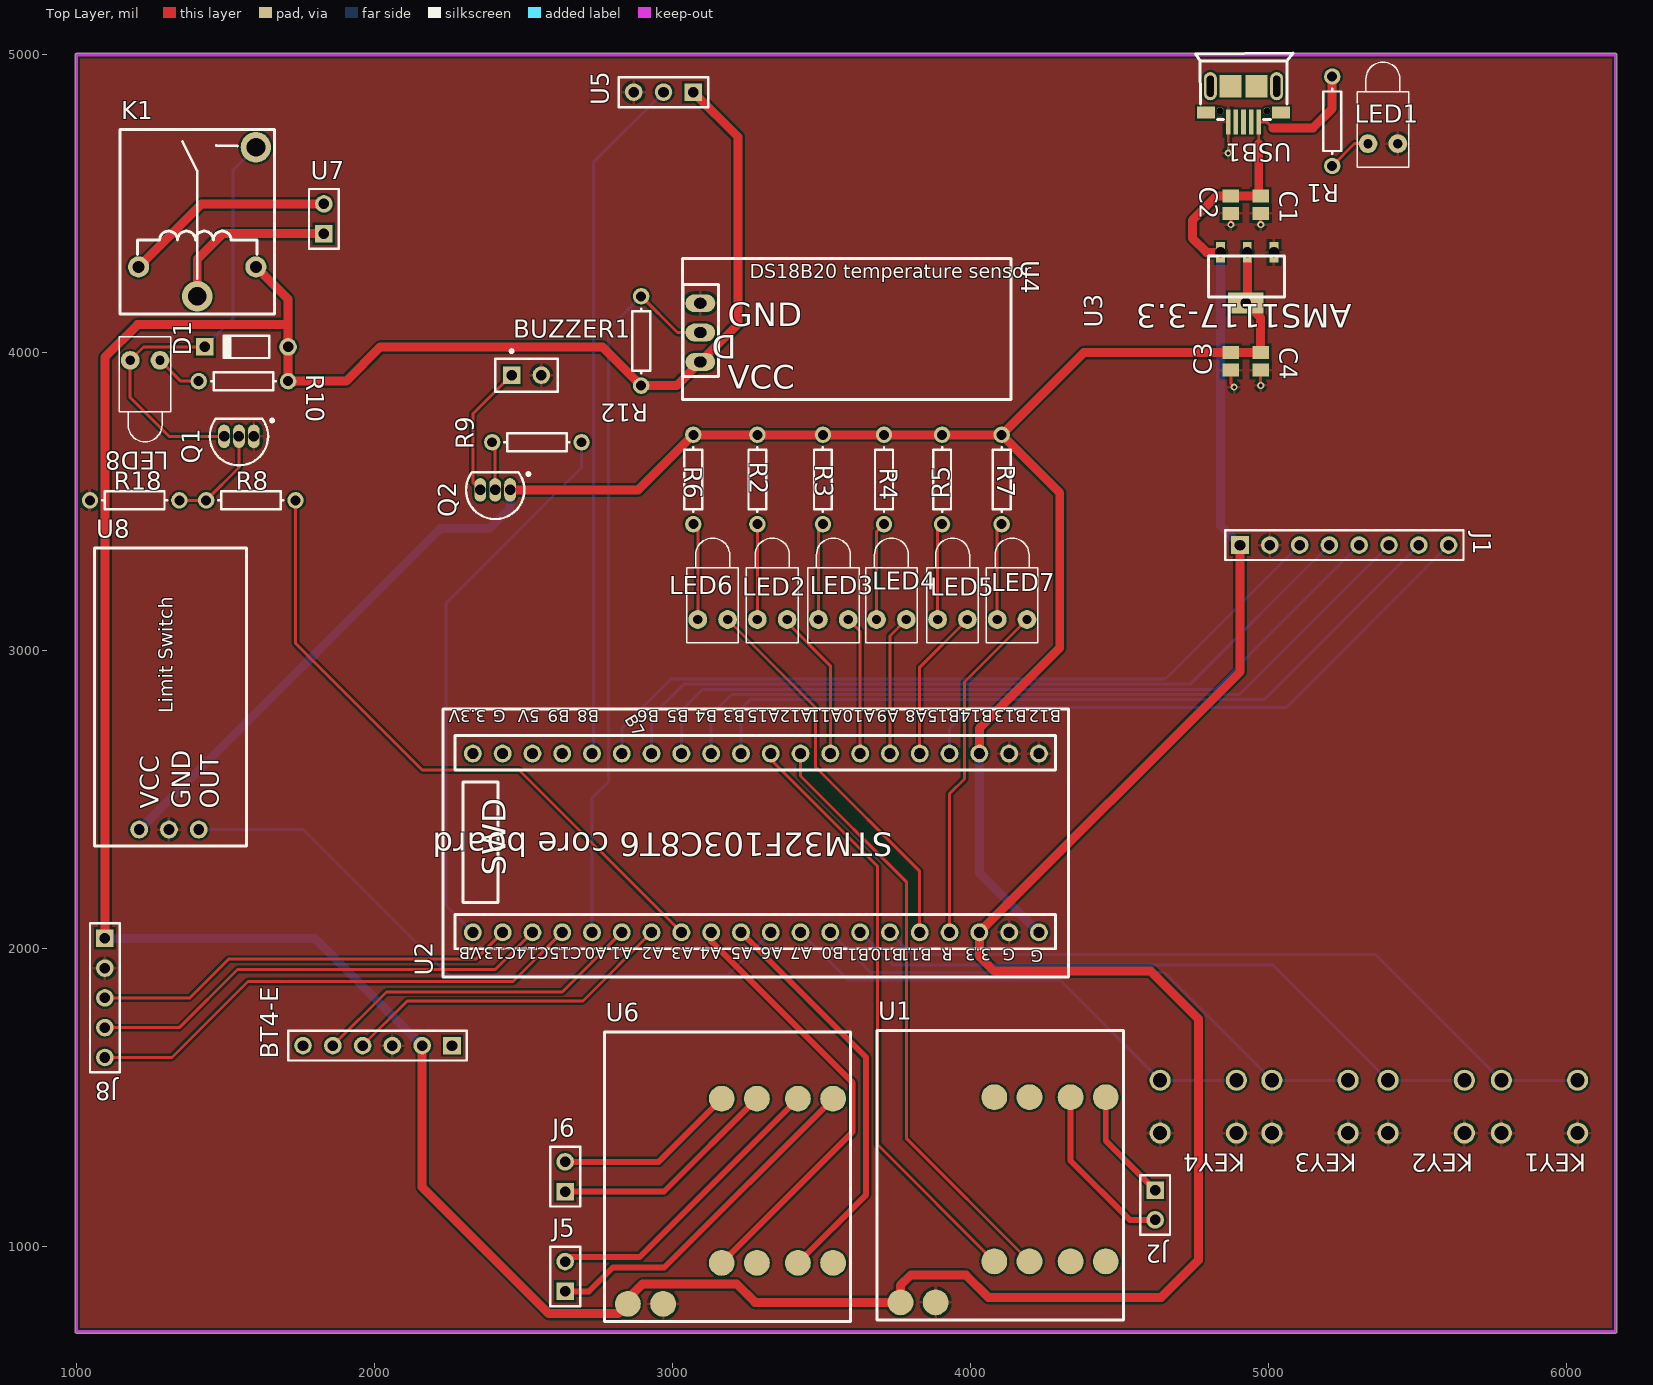
[diagram p0: Top Layer view]
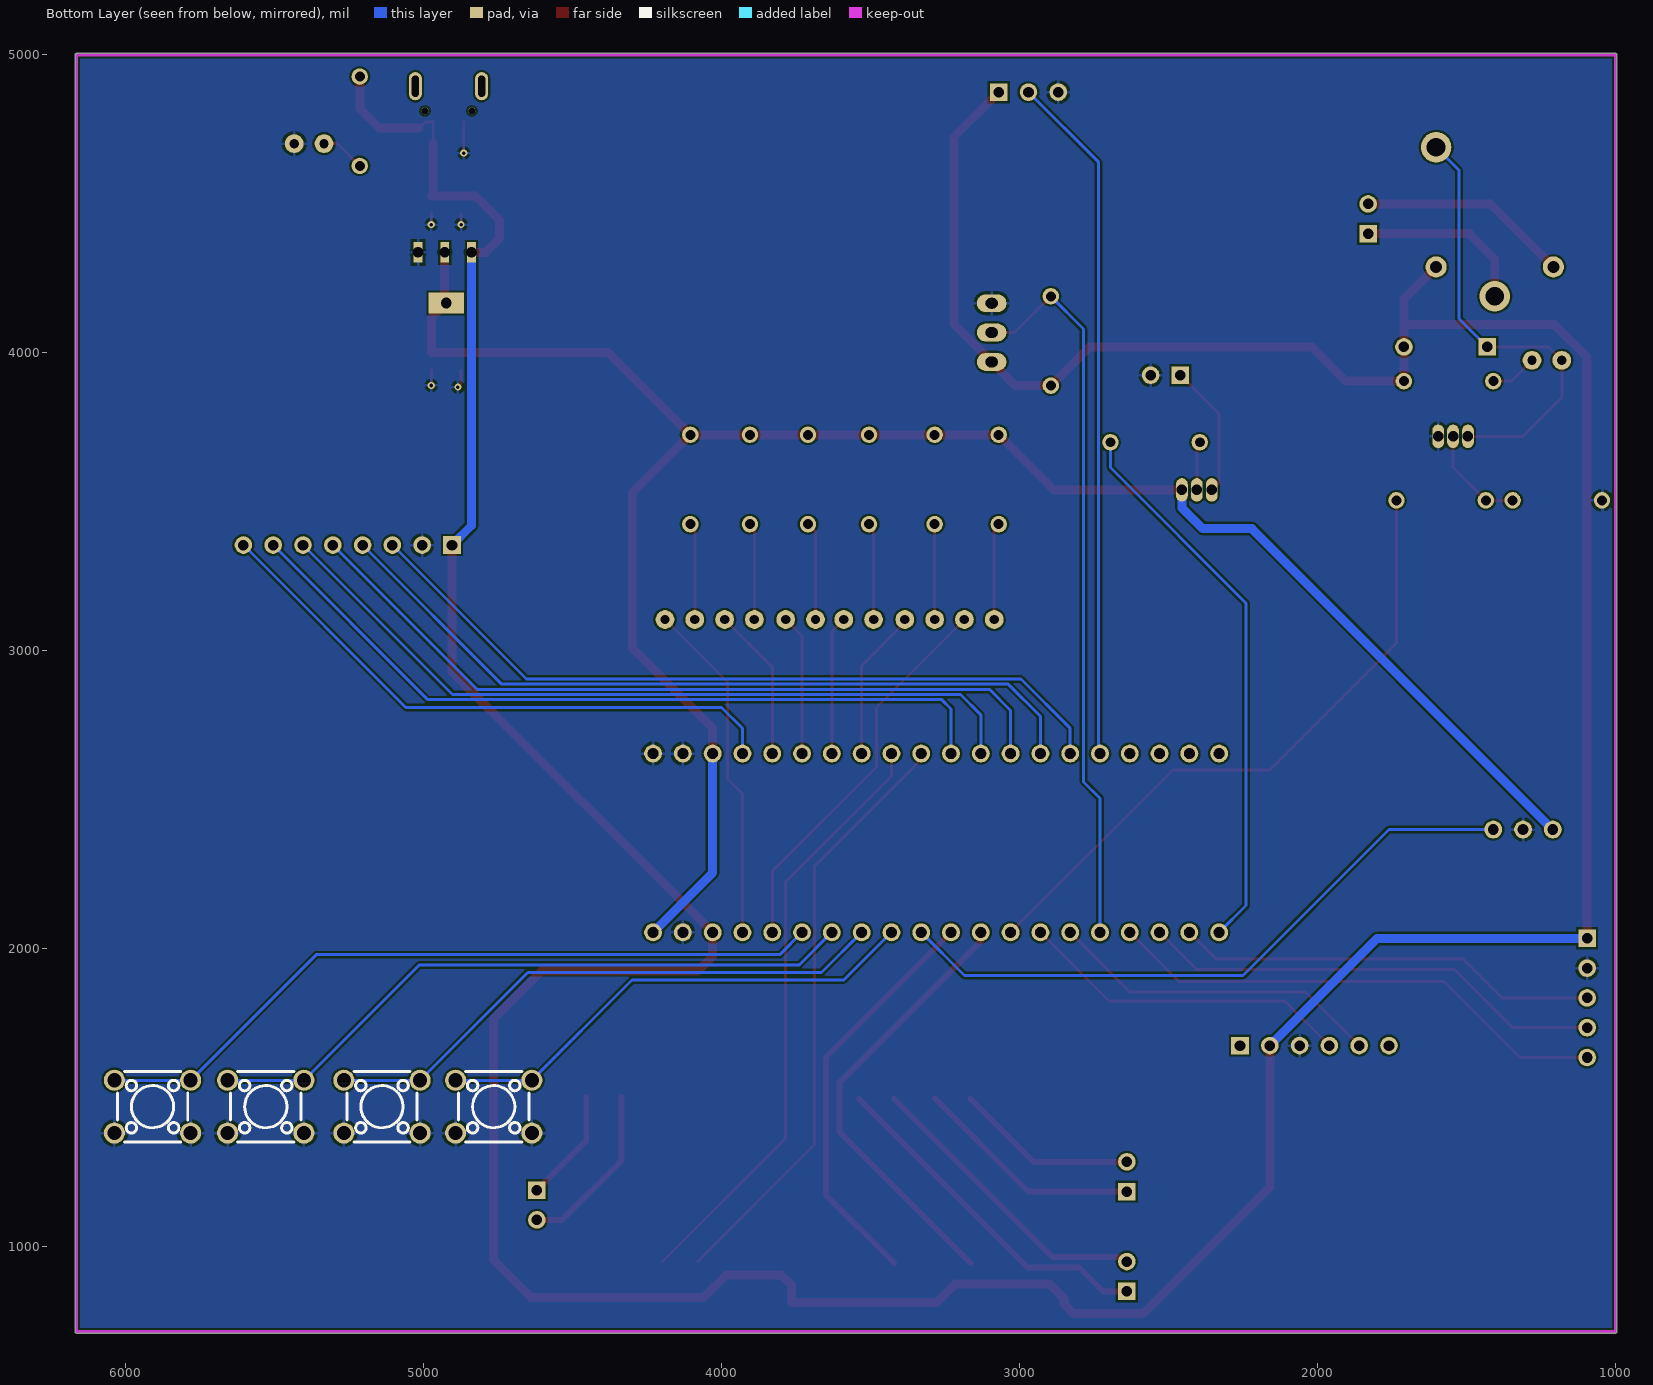
[diagram p1: Bottom Layer view, seen from below]
# Altium PCB MISC82193.PcbDoc
Units mil, origin at the board's own origin, x right, y up, seen from the top; angles counter-clockwise.
Board outline 5175.03 x 4295.03 mil, 2 copper layers (Top Layer, Bottom Layer); 48 components, 56 nets, 191 pads, 5 vias.

## Layer stack, top to bottom (the 12.6 mil dielectric is the usual default, probably not edited)
Top Solder: solder mask 0.4, Solder Resist, Dk 3.5
Top Layer: signal copper 1.4
Dielectric 1: dielectric 12.6, FR-4, Dk 4.8
Bottom Layer: signal copper 1.4
Bottom Solder: solder mask 0.4, Solder Resist, Dk 3.5

## Board outline
994.99,715 ccw(c1000,715) 1000,709.99 6165,709.99 ccw(c6165,715) 6170.02,715 6170.02,5000 ccw(c6165,5000) 6165,5005.02 1000,5005.02 ccw(c1000,5000) 994.99,5000

## Design rules (kind name [scope] priority, off if disabled: settings)
Clearance [All] p1: gap=7
MinimumSolderMaskSliver [All] p1: minsoldermaskwidth=0
PolygonConnect [All] p1: connectstyle=Relief reliefconductorwidth=10 reliefentries=4 polygonreliefangle="90 Angle" airgapwidth=10
RoutingVias [All] p1: holewidth=28 width=50 viastyle="Through Hole" minholewidth=28 minwidth=50 maxholewidth=28 maxwidth=50
SilkToSilkClearance [All] p1: silktosilkclearance=0
SilkToSolderMaskClearance [IsPad] p1: minsilkscreentomaskgap=0 clearancetoexposedcopper=TRUE
SolderMaskExpansion [All] p1: expansion=4
Width [All] p1: maxlimit=30 minlimit=10 preferedwidth=10
27 further rules are at their usual default settings.

## Components (designator, comment, footprint, x,y, rotation, side; value= is the part's Value field where it differs from the comment)
BT4-E "NO" HDR1X6 2260,1675 r180 top
BUZZER1 "5V" PIN2 2460,3925 r0 top
C1 "10uF" C0805 4974.45,4497.4 r270 top
C2 "100nF" C0805 4874.45,4497.4 r270 top
C3 "10uF" C0805 4874.45,3971.93 r90 top
C4 "100nF" C0805 4974.45,3971.93 r270 top
D1 "1N4148" DO-35 1570,4020 r180 top
J1 "HDR-M-2.54_1x8" HDR1X8 4905,3355 r0 top
J2 "HDR-M-2.54_1x2" HDR1X2 4620,1190 r270 top
J5 "HDR-M-2.54_1x2" HDR1X2 2640,850 r90 top
J6 "HDR-M-2.54_1x2" HDR1X2 2640,1185 r90 top
J8 "HDR-M-2.54_1x5" HDR1X5 1095,2035 r270 top
K1 "SRD-5VDC-SL-A" 012-1HW_BK 1405,4190 r90 top
KEY1 "K4-6×6_TH" 四脚轻触开关 5910,1470 r180 top
KEY2 "K4-6×6_TH" 四脚轻触开关 5530,1470 r180 top
KEY3 "K4-6×6_TH" 四脚轻触开关 5140,1470 r180 top
KEY4 "K4-6×6_TH" 四脚轻触开关 4765,1470 r180 top
LED1 "LED-TH-3mm_R" LED-1 5384.45,4702.4 r90 top
LED2 "LED-0603_R" LED-1 3335,3105 r90 top
LED3 "LED-0603_R" LED-1 3540,3105 r90 top
LED4 "LED-0603_R" LED-1 3735,3105 r90 top
LED5 "LED-0603_R" LED-1 3940,3105 r90 top
LED6 "LED-0603_R" LED-1 3135,3105 r90 top
LED7 "LED-0603_R" LED-1 4140,3105 r90 top
LED8 "LED-TH-3mm_R" LED-1 1230,3975 r270 top
Q1 "S8050-D" TO-92A 1545,3720 r90 top
Q2 "S8550" TO-92A 2405,3540 r90 top
R1 "4.7k" AXIAL-0.3 5214.45,4777.4 r270 top
R2 "1k" AXIAL-0.3 3285,3575 r270 top
R3 "1k" AXIAL-0.3 3505,3575 r270 top
R4 "1k" AXIAL-0.3 3710,3575 r270 top
R5 "1k" AXIAL-0.3 3905,3575 r270 top
R6 "1k" AXIAL-0.3 3070,3575 r270 top
R7 "1k" AXIAL-0.3 4105,3575 r270 top
R8 "1k" AXIAL-0.3 1585,3505 r180 top
R9 "1k" AXIAL-0.3 2545,3700 r180 top
R10 "4.7K" AXIAL-0.3 1560,3905 r0 top
R12 "4.7k" AXIAL-0.3 2895,4040 r270 top
R18 "10k" AXIAL-0.3 1195,3505 r0 top
U1 "1508S motor driver module" DIANJIQUDONG 4100,1240 r90 top
U2 "STM32F103C8T6 core board" STM32核心板 3056,3556.5 r90 top
U3 "AMS1117-3.3" AMS1117-3.3 5036.49,4227.13 r180 top
U4 "DS18B20" DS18B20 3585,4080 r0 top
U5 "NO" HDR1X3 3070,4875 r180 top
U6 "1508S motor driver module" DIANJIQUDONG 3185,1235 r90 top
U7 "Connect watering pump" HDR1X2 1830,4400 r90 top
U8 "NO" xianwei 1315,2845 r90 top
USB1 "MICRO5.9MMUSB" MICRO-USB-SMD_5P-P0.65-H-F_MICRO5.9MMUSB 4919.45,4872.4 r180 top

## Footprints (in the part's own frame and the unit in brackets; to place one, negate y for a bottom-side part, rotate by r counter-clockwise, add the part's x,y. Pads: shape width x height; smd on the part's side, far side on the other; paste and mask are expansions set on the pad)
012-1HW_BK [mm] "单刀单投/常开"
  round 1.8 hole 1: 1(2.5,5) 2(2.5,-5)
  round 2.6 hole 1.6: 3(0,0) 4(12.7,-5)
  silkscreen extent -1.52,-6.6 14.22,6.6, body extent -1.52,-6.1 13.98,6.1, height 12.9
AMS1117-3.3 [mm]
  rect 0.74x1.75 hole 0.914 paste+0 mask+0.051: 1(0.444,-2.801) 2(2.719,-2.801) 3(5.005,-2.801)
  rect 3x1.75 hole 0.914 paste+0 mask+0.051: 4(2.846,1.517)
  silkscreen extent -0.46,-2.49 6.04,1.01
AXIAL-0.3 [mm] "Axial Device, Thru-Hole; 2 Leads; 0.3 in Pin Spacing"
  round 1.4 hole 0.85: 1(-3.81,0) 2(3.81,0)
  silkscreen extent -2.77,-0.76 2.77,0.76
C0805 [mm] "Chip Capacitor, Body 2.0x1.3mm, IPC High Density"
  rect 1.1x1.4 smd: 1(-0.75,0) 2(0.75,0)
  body extent -1.1,-0.72 1.1,0.72, height 1.4
DIANJIQUDONG [mm]
  round 2.2 smd paste+0.102 mask+0.102: 1(-10.85,8.5) 2(-10.85,5.5) 3(-7.35,0.5) 4(-7.35,-2.5) 5(-7.35,-6) 6(-7.35,-9) 7(6.65,0.5) 8(6.65,-2.5) 9(6.65,-6) 10(6.65,-9)
  silkscreen extent -12.35,-10.5 12.35,10.5
DO-35 [mm] "Diode, Axial; Body 3.8 x 1.9 mm (LxDia. max), Lead Dia. 0.53 mm (max)"
  round 1.5 hole 0.9: 1(-3.55,0)
  rect 1.5x1.5 hole 0.9: 2(3.55,0)
  silkscreen extent -1.95,-0.95 2.05,0.95
DS18B20 [mil]
  oval 99.37x60 hole 35.43 slot 41.34 at 0 deg paste+0 mask+4: 1(-491.35,86.55) 2(-491.35,-11.88) 3(-491.35,-110.3)
  silkscreen extent -551,-236 551,236
HDR1X2 [mm] "Connector; Header; 2 Position"
  rect 1.5x1.5 hole 0.9: 1(0,0)
  round 1.5 hole 0.9: 2(2.54,0)
  silkscreen extent -1.27,-1.27 3.81,1.27
HDR1X3 [mm] "Connector; Header; 3 Position"
  rect 1.5x1.5 hole 0.9: 1(0,0)
  round 1.5 hole 0.9: 2(2.54,0) 3(5.08,0)
  silkscreen extent -1.27,-1.27 6.35,1.27
HDR1X5 [mm] "Connector; Header; 5 Position"
  rect 1.5x1.5 hole 0.9: 1(0,0)
  round 1.5 hole 0.9: 2(2.54,0) 3(5.08,0) 4(7.62,0) 5(10.16,0)
  silkscreen extent -1.27,-1.27 11.43,1.27
HDR1X6 [mm] "Connector; Header; 6 Position"
  rect 1.5x1.5 hole 0.9: 1(0,0)
  round 1.5 hole 0.9: 2(2.54,0) 3(5.08,0) 4(7.62,0) 5(10.16,0) 6(12.7,0)
  silkscreen extent -1.27,-1.27 13.97,1.27
HDR1X8 [mm] "Connector; Header; 8 Position"
  rect 1.5x1.5 hole 0.9: 1(0,0)
  round 1.5 hole 0.9: 2(2.54,0) 3(5.08,0) 4(7.62,0) 5(10.16,0) 6(12.7,0) 7(15.24,0) 8(17.78,0)
  silkscreen extent -1.27,-1.27 19.05,1.27
LED-1 [mm] "LED; 2 Leads"
  round 1.6 hole 0.8: 1(0,1.27) 2(0,-1.27)
  silkscreen extent -2,-2.2 6.95,2.2
MICRO-USB-SMD_5P-P0.65-H-F_MICRO5.9MMUSB [mm]
  rect 0.4x2.1 smd paste-100 mask+0.05: 1(-1.23,2.476) 2(-0.58,2.476) 3(0.07,2.476) 4(0.72,2.476) 5(1.37,2.476)
  rect 1.5x1 smd paste-100 mask+0.05: 6(-3.13,1.676) 6(3.27,1.676)
  oval 1.1x2.4 hole 0.6 slot 1.8 at 90 deg paste+0 mask+0.051: 6(-2.755,-0.574) 6(2.895,-0.574)
  rect 1.9x1.9 smd paste-100 mask+0.051: 6(-1.03,-0.574) 6(1.17,-0.574)
  round 0.6 hole 0.6 unplated paste+0: ""(-1.93,1.526) ""(2.07,1.526)
  silkscreen extent -4.16,-3.4 4.16,2.28
PIN2 [mm] "Photosensitive Diode; 2 Leads"
  rect 1.5x1.5 hole 0.9: 1(0,0)
  round 1.5 hole 0.9: 2(2.54,0)
  silkscreen extent -1.4,-1.4 3.94,2.17
STM32核心板 [mil]
  round 60 hole 36 slot 36.2 at 0 deg paste+0 mask+2: 1(-1501.5,726) 2(-1501.5,626) 3(-1501.5,526) 4(-1501.5,426) 5(-1501.5,326) 6(-1501.5,226) 7(-1501.5,126) 8(-1501.5,26) 9(-1501.5,-74) 10(-1501.5,-174) 11(-1501.5,-274) 12(-1501.5,-374) 13(-1501.5,-474) 14(-1501.5,-574) 15(-1501.5,-674) 16(-1501.5,-774) 17(-1501.5,-874) 18(-1501.5,-974) 19(-1501.5,-1074) 20(-1501.5,-1174) 21(-901.5,-1174) 22(-901.5,-1074) 23(-901.5,-974) 24(-901.5,-874) 25(-901.5,-774) 26(-901.5,-674) 27(-901.5,-574) 28(-901.5,-474) 29(-901.5,-374) 30(-901.5,-274) 31(-901.5,-174) 32(-901.5,-74) 33(-901.5,26) 34(-901.5,126) 35(-901.5,226) 36(-901.5,326) 37(-901.5,426) 38(-901.5,526) 39(-901.5,626) 40(-901.5,726)
  silkscreen extent -1652,-1274 -751,826
TO-92A [mm] "TO, Flat Index; 3 In-Line, Axial Leads; Body Dia. 4.5mm; Leads 0.51 x 0.48 mm (max)"
  oval 2x1 hole 0.9: 1(0,-1.27) 2(0,0) 3(0,1.27)
  silkscreen extent -2.48,-2.96 1.5,2.48, body extent -2.48,-2.5 1.5,2.5, height 6.86
xianwei [mil]
  round 60 hole 36 paste+4 mask+2: 1(-445,105) 2(-445,5) 3(-445,-95)
  silkscreen extent -500,-255 500,255
四脚轻触开关 [mm]
  round 1.8 hole 1.2 paste+0 mask+0.102: 1(3.25,2.25) 2(-3.25,2.25) 3(3.25,-2.25) 4(-3.25,-2.25)

## Part data
U1 U6: library part 电机驱动1508S模块
U2: library part STM32F103C8T6核心板
U7: library part 接浇水水泵

## Via types
v1: diameter 24, hole 12, Top Layer to Bottom Layer, 5 vias

## Nets (pads, with @x,y where several pads share a name; then routed paths per layer and width w, separated by ;. In a path a pad name is that pad's centre, name@x,y a point inside that pad or via, vN(x,y) a via of type N, cw(c..) or ccw(c..) an arc to the next point about the centre after c; other vN are vias at no path point)
+3.3V: C3.2 C4.1 Q2.1 R2.1 R3.1 R4.1 R5.1 R6.1 R7.1 U2.20 U2.23 U3.2 U3.4 U8.1 | length 6767.1
  Top Layer w30: Q2.1 2885,3540 R6.1 R2.1 R3.1 R4.1 R5.1 R7.1 ; U2.23 4030,2740 4300,3010 4300,3530 R7.1 ; U3.2 4929.45,4172.4 U3.4 4974.45,4117.4 C4.1 C3.2 4381.46,4001.46 R7.1
  Bottom Layer w30: U8.1 2220,3410 2385,3410 2455,3480 Q2.1 ; U2.23 4030,2255 U2.20
+5V: BT4-E.2 C1.1 C2.1 D1.1 J1.1 J8.1 K1.2 R1.1 R10.2 R12.2 U1.1 U2.18 U3.3 U4.3 U5.1 U6.1 USB1.1 | length 15740.5
  Top Layer w10: 4967.87,4702.87 USB1.1 4995.08,4774.92 5015,4755
  Top Layer w30: J8.1 1095,3985 1205,4095 1709.76,4095 ; K1.2 1709.76,4180.51 1709.76,4095 ; BT4-E.2 2160,1200 2585,775 2817.52,775 U6.1 2850.36,825.36 2900,875 3215,875 3277.16,812.84 U1.1 3765.36,870.36 3800,905 3985,905 4060,830 4640,830 4765,955 4765,1765 4605,1925 4080,1925 4030,1975 U2.18 4905,2930 J1.1 ; U5.1 3220,4725 3220,4096.05 U4.3 3013.95,3890 R12.2 2765,4020 2020,4020 1905,3905 R10.2 1710,4019.76 D1.1 1709.76,4095 ; U3.3 4792.6,4337.4 4745,4385 4745,4445 4826.93,4526.93 C2.1 C1.1 4967.87,4533.5 4967.87,4702.87 ; 5015,4755 5150,4755 5214.45,4819.45 R1.1
  Bottom Layer w30: J8.1 1800,2035 BT4-E.2 ; U3.3 4839.45,3420.55 J1.1
GND: BT4-E.3 BUZZER1.2 C1.2 C2.2 C3.1 C4.2 J1.2 J8.2 KEY1.1 KEY1.2 KEY2.1 KEY2.2 KEY3.1 KEY3.2 KEY4.1 KEY4.2 LED1.2 Q1.1 R18.1 U1.2 U2.19 U2.21 U2.22 U3.1 U4.1 U5.3 U6.2 U8.2 USB1.5 | length 292.7
  Top Layer w10: v1(4865.51,4670.51) USB1.5 ; C3.1 4874.45,3895.55 v1(4885,3885) ; v1(4874.45,4430.55) C2.2 ; v1(4974.45,3890.55) C4.2 ; v1(4974.45,4430.55) C1.2
INT1: K1.3 U7.1 | length 585.2
  Top Layer w30: K1.3 1405,4315 1490,4400 U7.1
NetBUZZER1_1: BUZZER1.1 Q2.3 | length 449.2
  Top Layer w10: Q2.3 2330,3565 2330,3795 BUZZER1.1
NetD1_2: D1.2 K1.4 LED8.2 Q1.3 | length 1503.8
  Top Layer w10: D1.2 1225,4020 LED8.2 1180,3850 1310,3720 Q1.3
  Bottom Layer w10: D1.2 1525,4114.76 1525,4613.15 K1.4
NetJ2_1: J2.1 U1.10 | length 380.4
  Top Layer w20: U1.10 4454.33,1355.67 J2.1
NetJ2_2: J2.2 U1.9 | length 579.1
  Top Layer w20: U1.9 4336.22,1288.78 4535,1090 J2.2
NetJ5_1: J5.1 U6.10 | length 1167.2
  Top Layer w20: J5.1 2720,850 2800,930 2972.52,930 U6.10
NetJ5_2: J5.2 U6.9 | length 1007.7
  Top Layer w20: J5.2 2655,965 2889.41,965 U6.9
NetJ6_1: J6.1 U6.8 | length 772.6
  Top Layer w20: J6.1 2971.61,1185 U6.8
NetJ6_2: J6.2 U6.7 | length 613
  Top Layer w20: J6.2 2953.51,1285 U6.7
NetK1_1: K1.1 U7.2 | length 709.5
  Top Layer w30: K1.1 1419.72,4500 U7.2
NetLED1_1: LED1.1 R1.2 | length 151.1
  Top Layer w10: R1.2 5289.45,4702.4 LED1.1
NetLED2_1: LED2.1 R2.2 | length 320
  Top Layer w10: LED2.1 R2.2
NetLED3_1: LED3.1 R3.2 | length 326.2
  Top Layer w10: LED3.1 3490,3410 R3.2
NetLED4_1: LED4.1 R4.2 | length 330.4
  Top Layer w10: LED4.1 3685,3400 R4.2
NetLED5_1: LED5.1 R5.2 | length 326.2
  Top Layer w10: LED5.1 3890,3410 R5.2
NetLED6_1: LED6.1 R6.2 | length 326.2
  Top Layer w10: R6.2 3085,3410 LED6.1
NetLED7_1: LED7.1 R7.2 | length 326.2
  Top Layer w10: LED7.1 4090,3410 R7.2
NetLED8_1: LED8.1 R10.1 | length 159
  Top Layer w10: LED8.1 1350,3905 R10.1
NetQ1_2: Q1.2 R8.2 R18.2 | length 350.6
  Top Layer w10: R18.2 R8.2 1545,3615 Q1.2
NetQ2_2: Q2.2 R9.2 | length 164.1
  Top Layer w10: R9.2 2405,3690 Q2.2
PA0: U2.36 U5.2 | length 2319.4
  Bottom Layer w10: U2.36 2734.56,2659.56 2734.56,4639.56 U5.2
PA1: J1.3 U2.35 | length 2614.7
  Bottom Layer w10: U2.35 2830,2740 2995,2905 4655,2905 J1.3
PA2: J1.4 U2.34 | length 2638.2
  Bottom Layer w10: U2.34 2930,2780 3038,2888 4738,2888 J1.4
PA3: J1.5 U2.33 | length 2649.9
  Bottom Layer w10: U2.33 3030,2800 3100,2870 4820,2870 J1.5
PA4: J1.6 U2.32 | length 2641.1
  Bottom Layer w10: U2.32 3130,2785 3198,2853 4903,2853 J1.6
PA5: J1.7 U2.31 | length 2652.8
  Bottom Layer w10: U2.31 3230,2805 3261,2836 4986,2836 J1.7
PA6: U1.3 U2.30 | length 2015.2
  Top Layer w10: U2.30 3330,2635 3688,2277 3688,1342.94 U1.3
PA7: U1.4 U2.29 | length 2022.7
  Top Layer w10: U2.29 3430,2580 3785,2225 3785,1364.06 U1.4
PA8: R12.1 U2.5 U4.2 | length 2452.5
  Top Layer w10: R12.1 3016.88,4068.12 U4.2
  Bottom Layer w10: U2.5 2730,2505 2785,2560 2785,4080 R12.1
PA9: BT4-E.5 U2.6 | length 1127.4
  Top Layer w10: BT4-E.5 2040,1855 2630,1855 U2.6
PA10: BT4-E.4 U2.7 | length 1127.4
  Top Layer w10: BT4-E.4 2110,1825 2700,1825 U2.7
PA11: R8.1 U2.8 | length 2176.8
  Top Layer w10: R8.1 1735,3025 2160,2600 2485,2600 U2.8
PA12: U2.9 U6.3 | length 1488.2
  Top Layer w20: U2.9 3130,2025 3605,1550 3605,1385.32 U6.3
PA15: U2.10 U6.5 | length 1378.1
  Top Layer w20: U2.10 3650,1635 3650,1174.41 U6.5
PB0: LED2.2 U2.28 | length 510.1
  Top Layer w10: LED2.2 3385,3095 3530,2950 U2.28
PB1: LED3.2 U2.27 | length 466.6
  Top Layer w10: LED3.2 3630,3065 U2.27
PB3: U2.11 U8.3 | length 2183
  Bottom Layer w10: U8.3 1760,2400 2250,1910 3185,1910 U2.11
PB4: KEY4.3 KEY4.4 U2.12 | length 1668.6
  Bottom Layer w10: U2.12 3590,1895 4300.63,1895 KEY4.3 KEY4.4
PB5: KEY3.3 KEY3.4 U2.13 | length 1943.6
  Bottom Layer w10: U2.13 3665,1920 4650.63,1920 KEY3.3 KEY3.4
PB6: KEY2.3 KEY2.4 U2.14 | length 2233.6
  Bottom Layer w10: U2.14 3740,1945 5015.63,1945 KEY2.3 KEY2.4
PB7: KEY1.3 KEY1.4 U2.15 | length 2513.6
  Bottom Layer w10: U2.15 3805,1980 5360.63,1980 KEY1.3 KEY1.4
PB8: LED6.2 U2.16 | length 1317.2
  Top Layer w10: LED6.2 3480,2810 3480,2610 3830,2260 U2.16
PB9: LED7.2 U2.17 | length 1157.7
  Top Layer w10: U2.17 3930,2520 3980,2570 3980,2895 LED7.2
PB10: LED4.2 U2.26 | length 472.8
  Top Layer w10: U2.26 3730,3050 LED4.2
PB11: LED5.2 U2.25 | length 516.3
  Top Layer w10: U2.25 3830,2945 LED5.2
PB12: R9.1 U2.1 | length 1870.7
  Bottom Layer w10: U2.1 2240,2145 2240,3160 2695,3615 R9.1
PB13: J8.3 U2.2 | length 1426.1
  Top Layer w10: J8.3 1380,1835 1510,1965 2340,1965 U2.2
PB14: J8.4 U2.3 | length 1567.5
  Top Layer w10: J8.4 1345,1735 1540,1930 2405,1930 U2.3
PB15: J8.5 U2.4 | length 1709
  Top Layer w10: J8.5 1320,1635 1575,1890 2465,1890 U2.4
PC13: U2.39
PC14: U2.38
PC15: U2.37
RST: J1.8 U2.24 | length 2014.7
  Bottom Layer w10: U2.24 3930,2740 4000,2810 5060,2810 J1.8
pads on no net: BT4-E.1 BT4-E.6 U1.5 U1.6 U1.7 U1.8 U2.40 U6.4 U6.6 USB1. USB1.2 USB1.3 USB1.4 USB1.6

## Polygon pours and split planes (outlines as drawn)
GND on Top Layer "G" (solid, remove dead copper, pour order 0): 635,5350 765,5220 6470,5220 6470,300 6425,255 6360,320 555,320
GND on Bottom Layer "G" (solid, remove dead copper, pour order 2): 890,390 6395,390 6465,320 6445,340 6445,5430 940,5430 535,5835

## Keep-outs
Keep-Out Layer:
  lines w10: 1000,765 1000,5000 6075,5000 ; 1000,775 1000,715 2865,715 6165,715 6165,5000 6035,5000